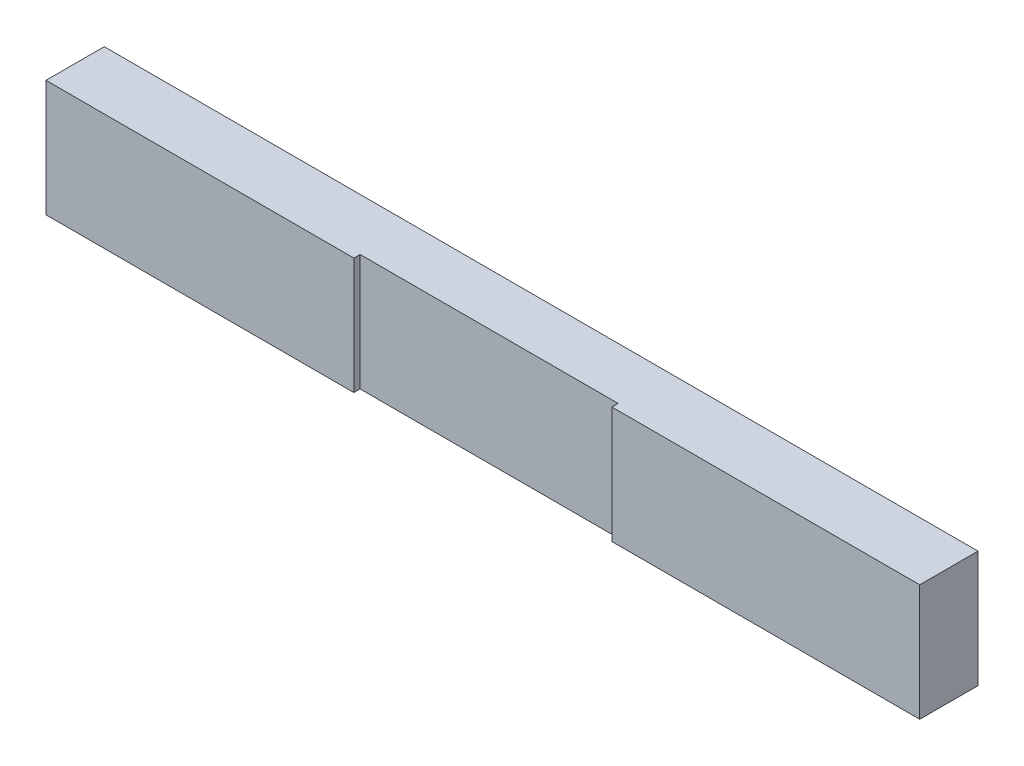
from build123d import *

# Parameters (mm, degrees)
SKETCH_1_W          = 210
SKETCH_1_H          = 28
EXTRUDE_1_DEPTH     = 14
SKETCH_2_W          = 62
SKETCH_2_H          = 28
CUT_EXTRUDE_1_DEPTH = 1.5


with BuildPart() as part:
    # 草图1 → 凸台-拉伸1 (new body)
    with BuildSketch(Plane.XY):
        Rectangle(SKETCH_1_W, SKETCH_1_H)
    extrude(amount=EXTRUDE_1_DEPTH)

    # 草图2 → 切除-拉伸1 (cut)
    with BuildSketch(Plane.XY.offset(14)):
        Rectangle(SKETCH_2_W, SKETCH_2_H)
    extrude(amount=-CUT_EXTRUDE_1_DEPTH, mode=Mode.SUBTRACT)


solid = part.part
